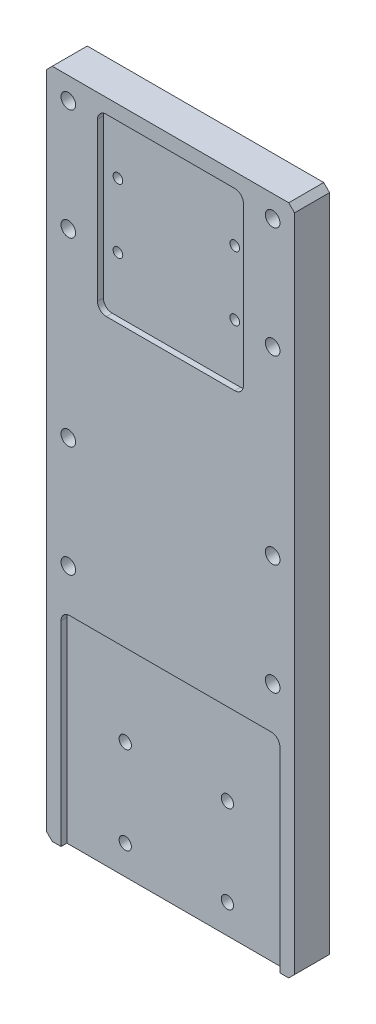
from build123d import *

# Parameters (mm, degrees)
SKETCH_2_W             = 85
SKETCH_2_H             = 230
EXTRUDE_1_DEPTH        = 12
CUT_EXTRUDE_2_DEPTH    = 2
HOLE_WIZARD_M5_1_D     = 4.2
HOLE_WIZARD_M4_1_D     = 3.3
HOLE_WIZARD_M6_1_D     = 5
HOLE_WIZARD_M6_1_DEPTH = 15
HOLE_WIZARD_M6_1_TIP   = 1.502151548
CHAMFER_1_SIZE         = 2


with BuildPart() as part:
    # 草图2 → 凸台-拉伸1 (new body)
    with BuildSketch(Plane.XY):
        Rectangle(SKETCH_2_W, SKETCH_2_H)
    extrude(amount=EXTRUDE_1_DEPTH)

    # 草图16 → 切除-拉伸2 (cut)
    with BuildSketch(Plane.XY.offset(12)):
        with BuildLine():
            Line((-22, 110), (22, 110))
            ThreePointArc((22, 110), (24.121320344, 109.121320344), (25, 107))
            Line((25, 107), (25, 53))
            ThreePointArc((25, 53), (24.121320344, 50.878679656), (22, 50))
            Line((22, 50), (-22, 50))
            ThreePointArc((-22, 50), (-24.121320344, 50.878679656), (-25, 53))
            Line((-25, 53), (-25, 107))
            ThreePointArc((-25, 107), (-24.121320344, 109.121320344), (-22, 110))
        make_face()
        with BuildLine():
            Line((-37.5, -115), (37.5, -115))
            Line((37.5, -115), (37.5, -48))
            ThreePointArc((37.5, -48), (36.621320344, -45.878679656), (34.5, -45))
            Line((34.5, -45), (-34.5, -45))
            ThreePointArc((-34.5, -45), (-36.621320344, -45.878679656), (-37.5, -48))
            Line((-37.5, -48), (-37.5, -115))
        make_face()
    extrude(amount=-CUT_EXTRUDE_2_DEPTH, mode=Mode.SUBTRACT)

    # M5 螺纹孔1 (through all)
    with Locations(Plane(origin=(0, 0, 0), x_dir=(-1, 0, 0), z_dir=(0, 0, -1))):
        with Locations((-17.5, -75), (17.5, -75), (17.5, -105), (-17.5, -105)):
            Hole(HOLE_WIZARD_M5_1_D / 2)

    # M4 螺纹孔1 (through all)
    with Locations(Plane.XY.offset(12)):
        with Locations((-20, 69), (20, 69), (-20, 91), (20, 91)):
            Hole(HOLE_WIZARD_M4_1_D / 2)

    # M6 螺纹孔1
    with Locations(Plane(origin=(0, 0, 0), x_dir=(-1, 0, 0), z_dir=(0, 0, -1))):
        with Locations((-35, 107.5), (-35, 69.5), (35, 69.5), (35, 107.5), (-35, 7.5), (-35, -30.5), (35, -30.5), (35, 7.5)):
            Hole(HOLE_WIZARD_M6_1_D / 2, depth=HOLE_WIZARD_M6_1_DEPTH)
            with Locations((0, 0, -(HOLE_WIZARD_M6_1_DEPTH + HOLE_WIZARD_M6_1_TIP / 2))):  # 118° drill point
                Cone(0, HOLE_WIZARD_M6_1_D / 2, HOLE_WIZARD_M6_1_TIP, mode=Mode.SUBTRACT)

    # 倒角1
    chamfer_1_edges = [part.edges().sort_by_distance(p)[0] for p in [
        (42.5, -115, 6),
        (-42.5, -115, 6),
        (-42.5, 115, 6),
        (42.5, 115, 6),
    ]]
    chamfer(chamfer_1_edges, length=CHAMFER_1_SIZE)


solid = part.part
